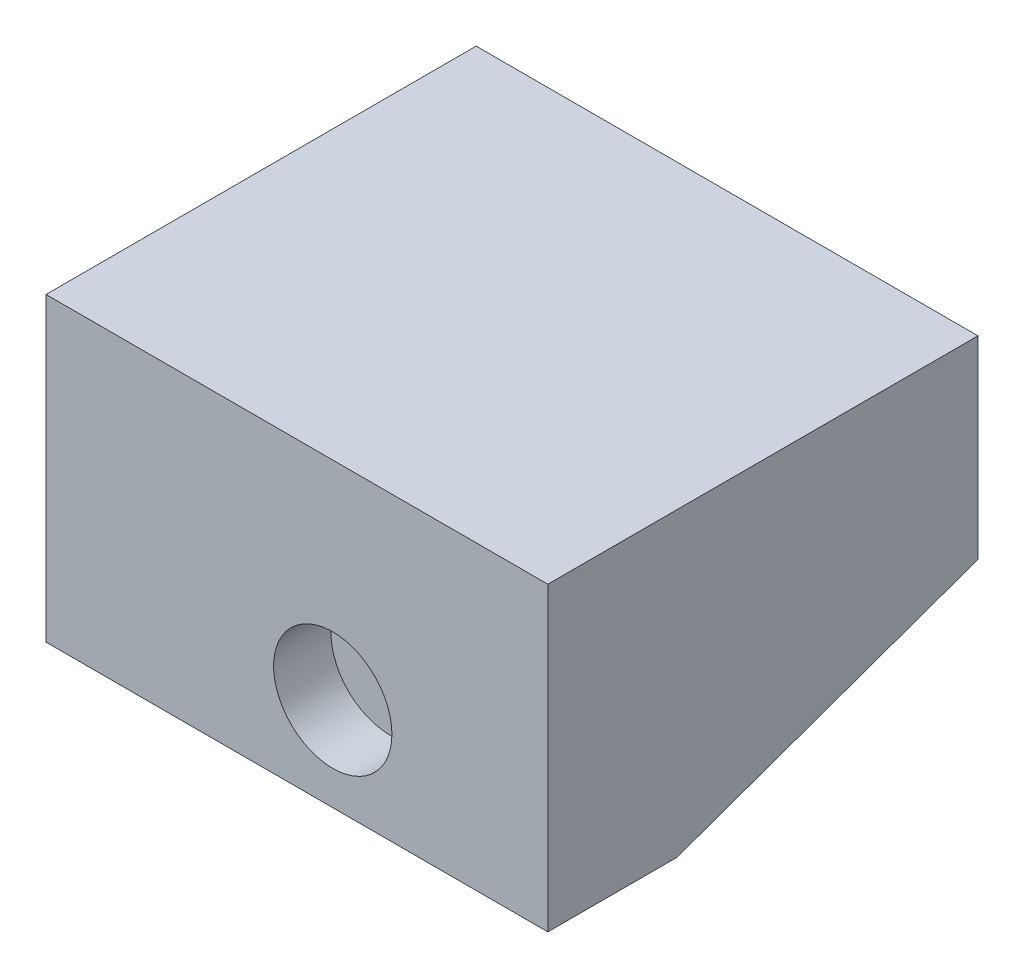
SolidWorks part; units mm, degrees
ref_plane "Front Plane" through (0, 0, 0) normal (0, 0, 1) x (1, 0, 0)
ref_plane "Top Plane" through (0, 0, 0) normal (0, 1, 0) x (1, 0, 0)
ref_plane "Right Plane" through (0, 0, 0) normal (1, 0, 0) x (0, 0, -1)
sketch "Sketch1" plane through (0, 0, 0) normal (0, 1, 0) x (1, 0, 0)
  line L1 (-30, 30) -> (30, 30)
  line L2 (-30, 30) -> (-30, -30)
  line L3 (-30, -30) -> (30, -30)
  line L4 (30, 30) -> (30, -30)
  line L5 (-30, 30) -> (30, -30) construction
  line L6 (-30, -30) -> (30, 30) construction
  point P0 (0, 0)
  dimension "D1" = 60
  dimension "D2" = 60
extrude "Boss-Extrude1" add sketch "Sketch1" along normal blind 20
sketch "Sketch2" plane through (30, 0, 0) normal (1, 0, 0) x (0, 0, -1)
  line L0 (30, 20) -> (30, 0)
  line L1 (30, 0) -> (30, -7)
  line L2 (30, -7) -> (-12, -22)
  line L3 (-12, -22) -> (-30, -22)
  line L4 (-30, -22) -> (-30, 20)
  line L5 (-30, 20) -> (30, 20)
  dimension "D1" = 42
  dimension "D2" = 18
  dimension "D3" = 27
extrude "Boss-Extrude2" add sketch "Sketch2" against normal blind 70
sketch "Sketch8" plane through (0, 0, 30) normal (0, 0, 1) x (1, 0, 0)
  line L0 (0, 22.3133) -> (0, -18.434) construction
  line L1 (-40, -22) -> (30, -22) construction
  circle A0 centre (0, -9) radius 8.25
  dimension "D1" = 16.5
  dimension "D2" = 13
extrude "Cut-Extrude5" cut sketch "Sketch8" against normal blind 8
